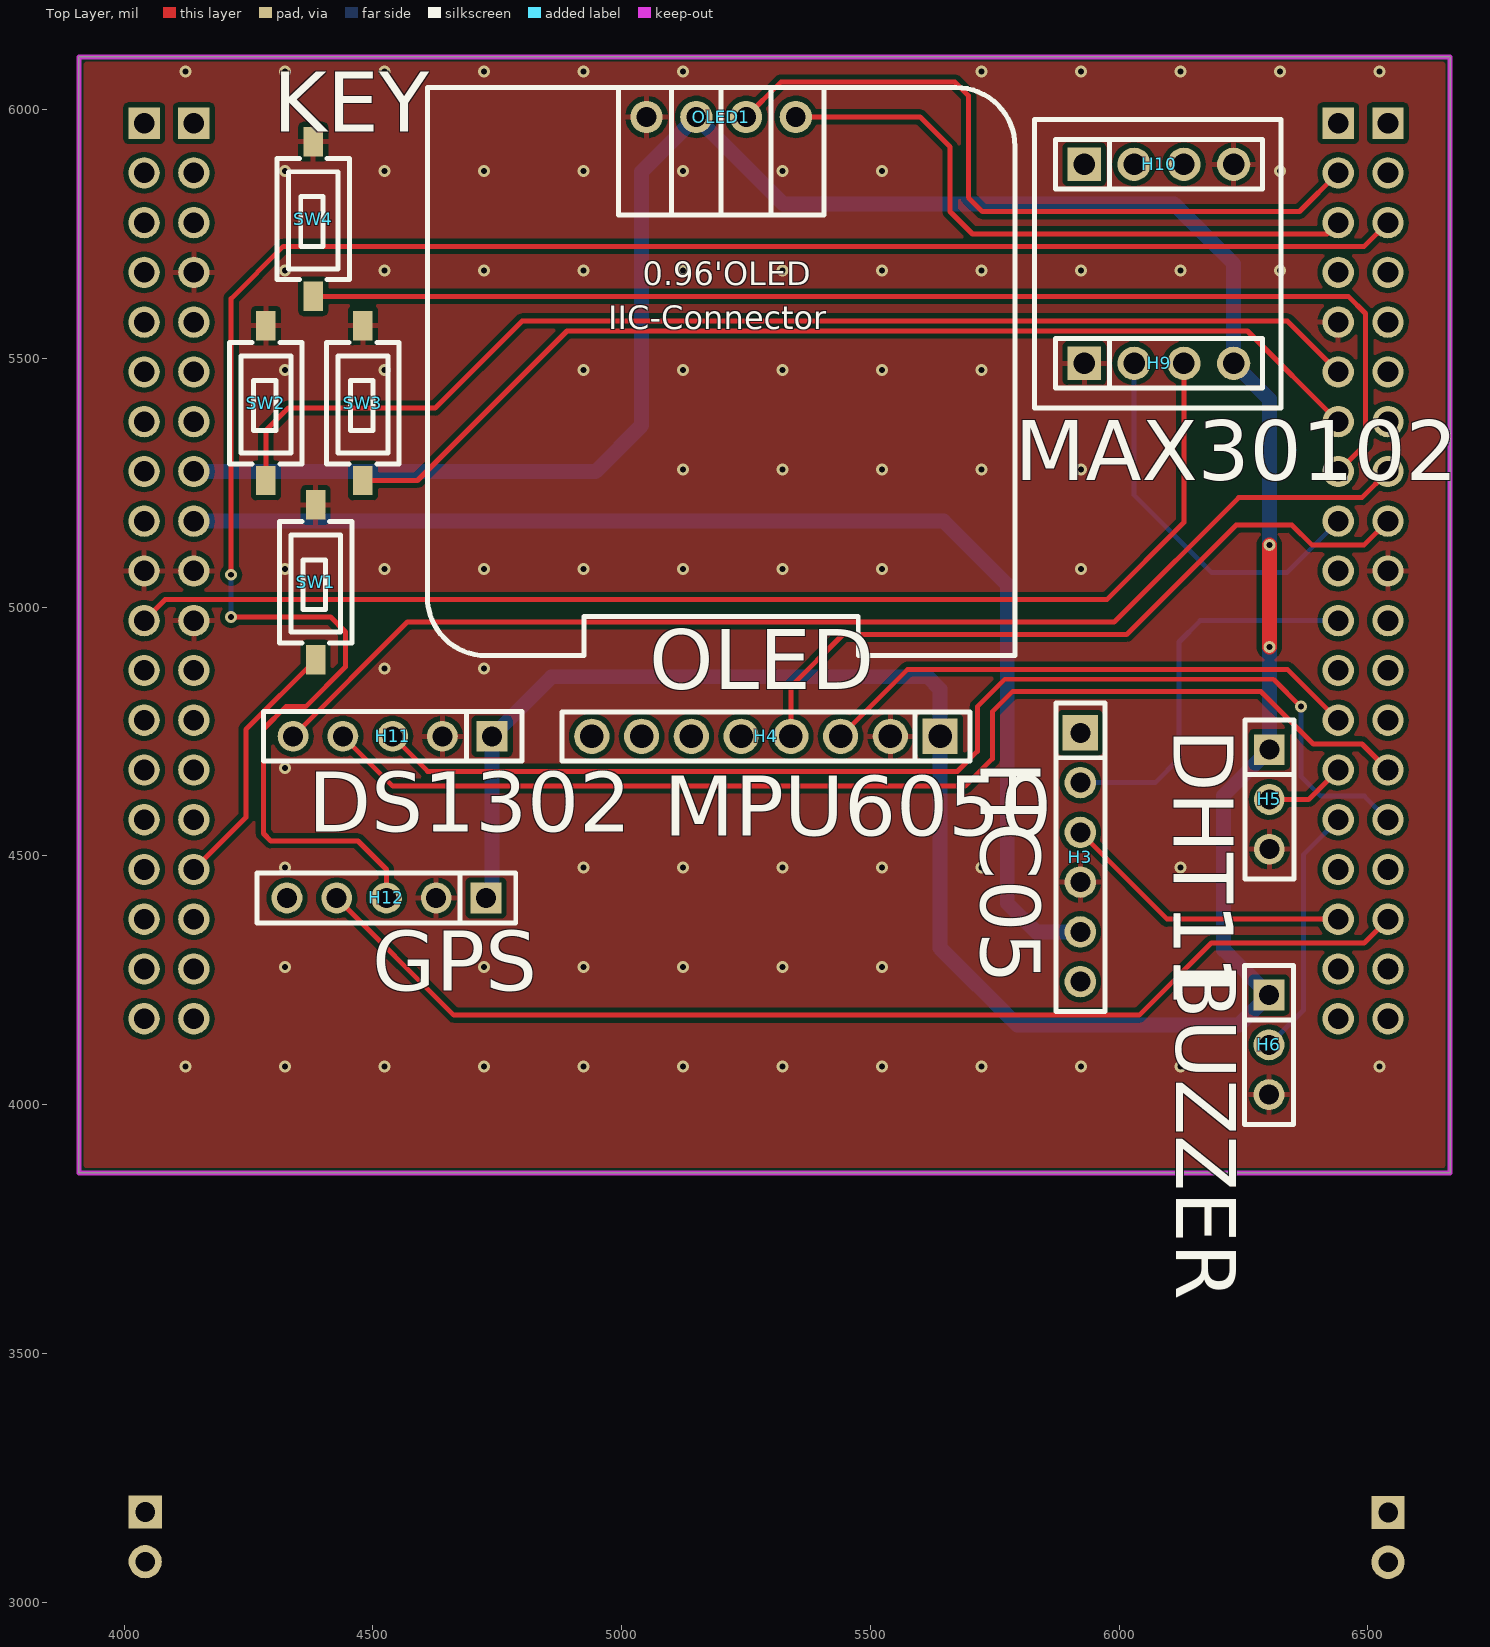
[diagram p0: Top Layer view]
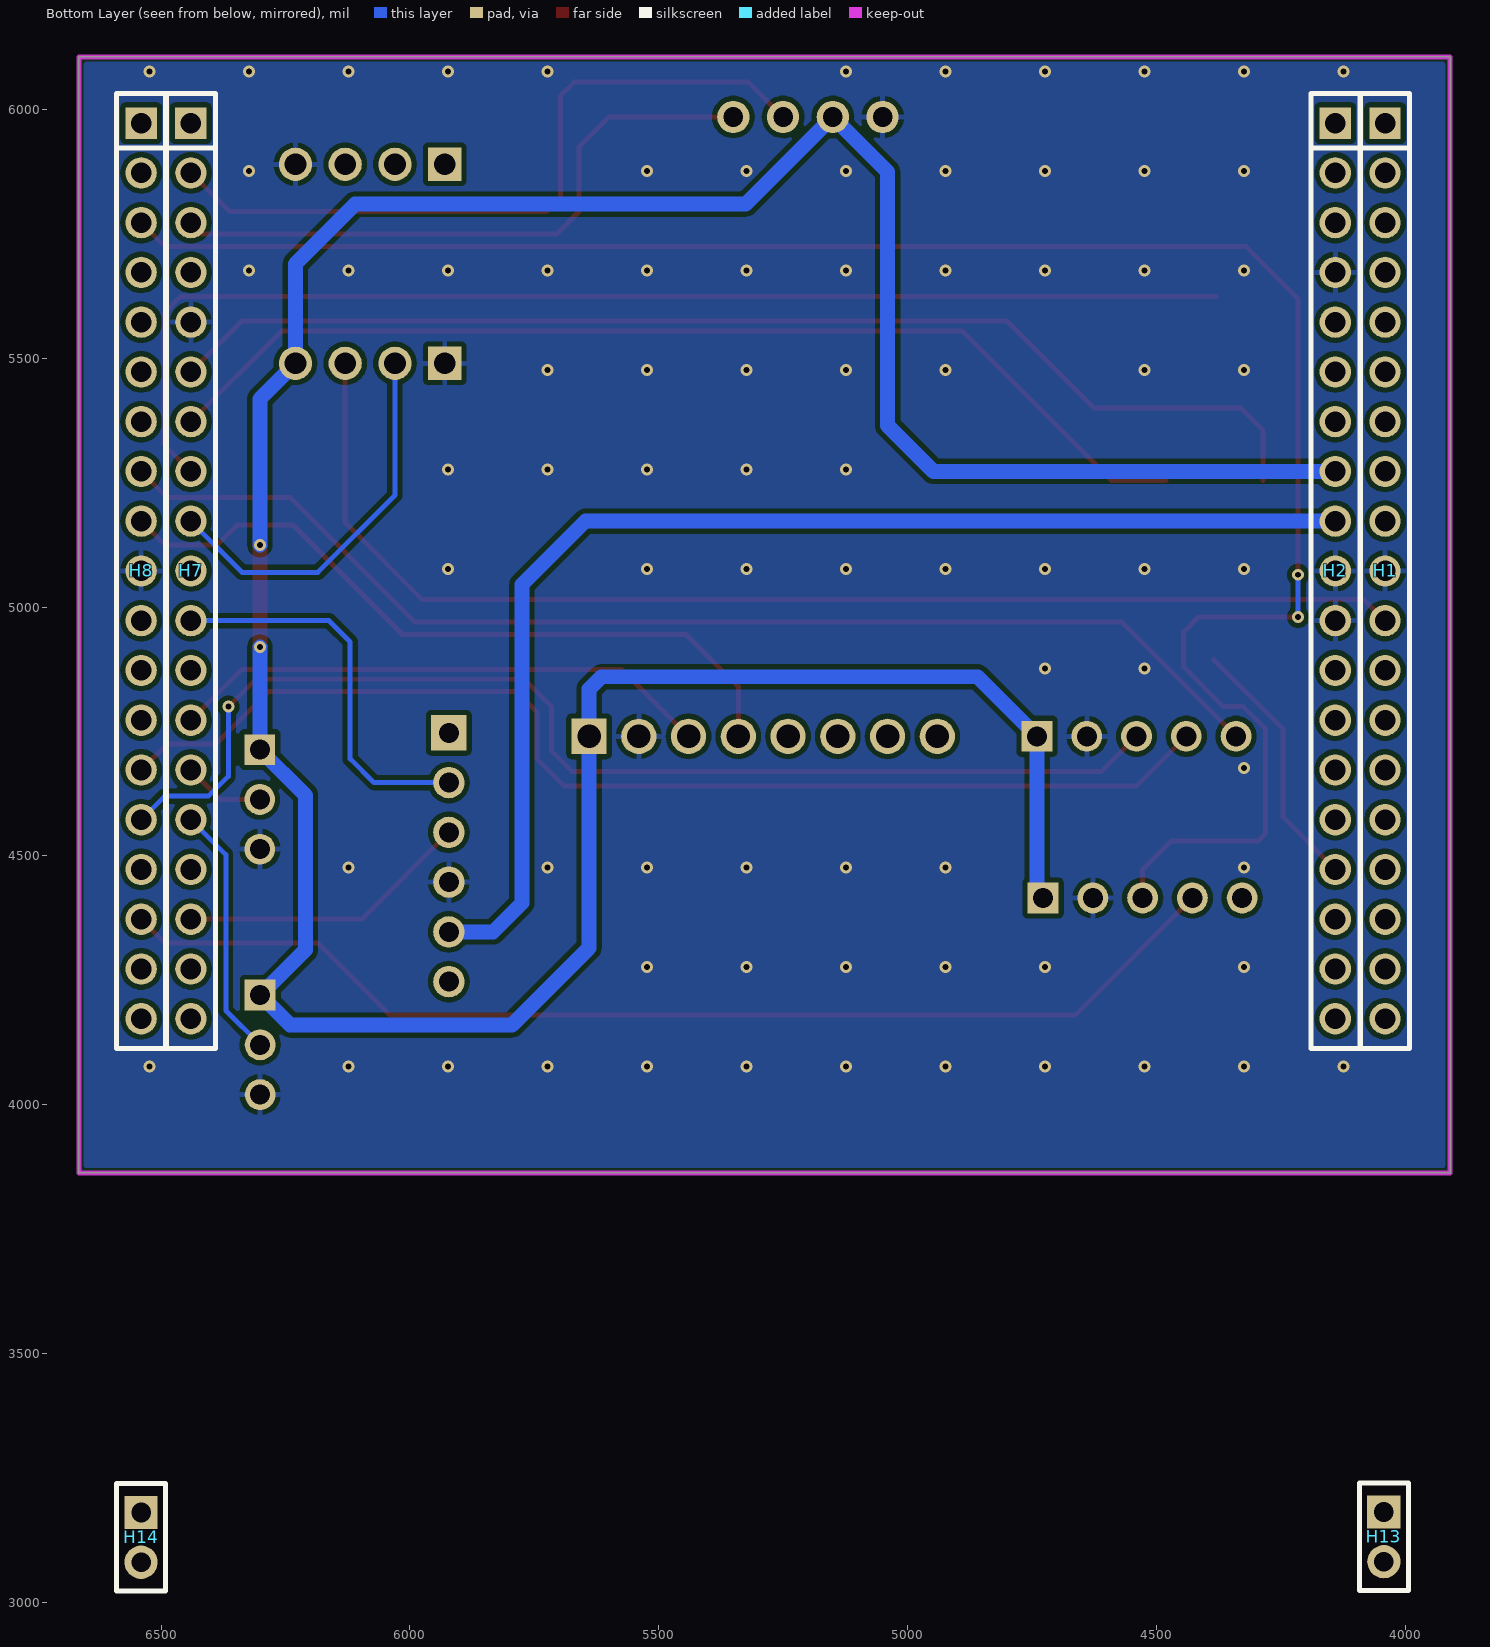
[diagram p1: Bottom Layer view, seen from below]
# Altium PCB MISC82907.pcbdoc
Units mil, origin at the board's own origin, x right, y up, seen from the top; angles counter-clockwise.
Board outline 2755.91 x 2243.03 mil, 2 copper layers (Top Layer, Bottom Layer), stack 62.206 mil thick; 19 components, 75 nets, 130 pads, 83 vias.

## Layer stack, top to bottom
Top Solder Mask Layer: solder mask 0.394, Dk 3.3
Top Layer: signal copper 1.379
Dielectric1: surface 59.449, FR4, Dk 4.5
Bottom Layer: signal copper 1.378
Bottom Solder Mask Layer: solder mask 0.394, Dk 3.3

## Board outline
6665.16,3862.65 6665.16,6105.69 3909.25,6105.69 3909.25,3862.65

## Design rules (kind name [scope] priority, off if disabled: settings)
BoardOutlineClearance copperThickness2oz_1 [All] p2 off: genericclearance=7.99 ignorepadtopadclearanceinfootprint=FALSE except(0: Arc-SplitContinuation Track-SplitContinuation SMDPad-SplitContinuation THPad-SplitContinuation Via-SplitContinuation Fill-SplitContinuation Region-SplitContinuation Poly-SplitContinuation Text-SplitContinuation Hole-SplitContinuation; 5.98: Arc-CutoutEdge SMDPad-CutoutEdge THPad-CutoutEdge Via-CutoutEdge Fill-CutoutEdge Region-CutoutEdge Text-CutoutEdge; 6.93: Hole-OutlineEdge Hole-CutoutEdge; 10: Poly-OutlineEdge Poly-CutoutEdge; 11.81: Arc-OutlineEdge Track-OutlineEdge SMDPad-OutlineEdge THPad-OutlineEdge Via-OutlineEdge Fill-OutlineEdge Region-OutlineEdge Text-OutlineEdge Track-CutoutEdge)
BoardOutlineClearance copperThickness1oz_1 [All] p4: genericclearance=4.02 ignorepadtopadclearanceinfootprint=FALSE except(0: Arc-SplitContinuation Track-SplitContinuation SMDPad-SplitContinuation THPad-SplitContinuation Via-SplitContinuation Fill-SplitContinuation Region-SplitContinuation Poly-SplitContinuation Text-SplitContinuation Hole-SplitContinuation; 6: SMDPad-CutoutEdge THPad-CutoutEdge Via-CutoutEdge Fill-CutoutEdge Region-CutoutEdge Text-CutoutEdge; 6.93: Hole-OutlineEdge Hole-CutoutEdge; 10: Poly-OutlineEdge Poly-CutoutEdge; 11.8: Arc-OutlineEdge Track-OutlineEdge SMDPad-OutlineEdge THPad-OutlineEdge Via-OutlineEdge Fill-OutlineEdge Region-OutlineEdge Text-OutlineEdge; 11.81: Arc-CutoutEdge Track-CutoutEdge)
Clearance copperThickness2oz [All] p1 off: gap=7.99 ignorepadtopadclearanceinfootprint=FALSE except(5.98: SMDPad-Track SMDPad-SMDPad THPad-Track SMDPad-THPad THPad-THPad Track-Via SMDPad-Via THPad-Via Via-Via Fill-Track Region-Track Fill-SMDPad Region-SMDPad Fill-THPad Region-THPad Fill-Via Region-Via Fill-Fill Fill-Region Region-Region Arc-Track Arc-SMDPad Arc-THPad Arc-Via Fill-Arc Region-Arc Arc-Arc Text-Track SMDPad-Text Text-THPad Text-Via Fill-Text Region-Text Arc-Text Text-Text; 6.93: Hole-Track Hole-SMDPad Hole-THPad Hole-Via Fill-Hole Region-Hole Hole-Arc Hole-Text; 10: Poly-Track Poly-SMDPad Poly-THPad Poly-Via Poly-Fill Poly-Region Poly-Poly Poly-Arc Poly-Text Poly-Hole)
Clearance copperThickness1oz [All] p3: gap=4.02 ignorepadtopadclearanceinfootprint=FALSE except(5.98: SMDPad-Track SMDPad-SMDPad THPad-Track SMDPad-THPad THPad-THPad Track-Via SMDPad-Via THPad-Via Via-Via Fill-Track Region-Track Fill-SMDPad Region-SMDPad Fill-THPad Region-THPad Fill-Via Region-Via Fill-Fill Fill-Region Region-Region; 6: Arc-Track Arc-SMDPad Arc-THPad Arc-Via Fill-Arc Region-Arc Arc-Arc Text-Track SMDPad-Text Text-THPad Text-Via Fill-Text Region-Text Arc-Text Text-Text; 6.93: Hole-Track Hole-SMDPad Hole-THPad Hole-Via Fill-Hole Region-Hole Hole-Arc Hole-Text; 10: Poly-Track Poly-SMDPad Poly-THPad Poly-Via Poly-Fill Poly-Region Poly-Poly Poly-Arc Poly-Text Poly-Hole)
DiffPairsRouting differentialPair [All] p1: maxlimit=6 minlimit=6 mostfreqgap=6 toplayer_minwidth=5 toplayer_prefwidth=10 toplayer_maxwidth=100 toplayer_mingap=6 toplayer_prefgap=6 toplayer_maxgap=6 bottomlayer_minwidth=5 bottomlayer_prefwidth=10 bottomlayer_maxwidth=100 bottomlayer_mingap=6 bottomlayer_prefgap=6 bottomlayer_maxgap=6 maxuncoupledlength=10
HoleToHoleClearance otherClearance [All] p1: gap=11.81 allowstackedmicrovias=TRUE
Length netLength [All] p1: minlimit=0 maxlimit=0
MatchedLengths netLengthTolerance [All] p1: tolerance=1000
PasteMaskExpansion pasteMaskExpansion [All] p1: expansion=0
PlaneConnect innerPlane [All] p1: planeconnectstyle=Relief reliefexpansion=20 reliefentries=4 reliefconductorwidth=10 reliefairgap=10
PolygonConnect copperRegion [(InNet('GND'))] p1: connectstyle=Relief reliefconductorwidth=10 reliefentries=4 polygonreliefangle="90 Angle" airgapwidth=10 via.connectstyle=Relief via.reliefconductorwidth=10 via.reliefentries=4 via.polygonreliefangle="90 Angle" via.airgapwidth=10
RoutingVias viaSize [All] p1: holewidth=12.01 width=24.02 viastyle="Through Hole" minholewidth=11.81 minwidth=19.68 maxholewidth=248.03 maxwidth=393.7
SolderMaskExpansion solderMaskExpansion [IsVia] p1: expansion=-1000 istentingtop=TRUE
SolderMaskExpansion solderMaskExpansion [All] p2: expansion=2 istentingtop=FALSE
Width copperThickness2oz_2 [All] p1 off: maxlimit=100 minlimit=8 preferedwidth=10
Width copperThickness1oz_2 [All] p2: maxlimit=100 minlimit=5 preferedwidth=10

## Components (designator, comment, footprint, x,y, rotation, side; value= is the part's Value field where it differs from the comment)
H1 "C2897382" HDR-TH_19P-P2.54-V-F 4040.16,5072.65 r270 bottom locked
H2 "C2897382" HDR-TH_19P-P2.54-V-F 4140.16,5072.65 r270 bottom locked
H3 "" HDR-TH_6P-P2.54-V-F 5921.75,4497.21 r270 top
H4 "" HDR-TH_8P-P2.54-V-F-1 5290,4740.21 r180 top
H5 "" HDR-TH_3P-P2.54-V-F 6301.67,4613.38 r270 top
H6 "" HDR-TH_3P-P2.54-V-F 6300.99,4120.2 r270 top
H7 "C2897382" HDR-TH_19P-P2.54-V-F 6440.16,5072.65 r270 bottom locked
H8 "C2897382" HDR-TH_19P-P2.54-V-F 6540.16,5072.65 r270 bottom locked
H9 "" HDR-TH_4P-P2.54-V-F 6080,5490 r0 top
H10 "" HDR-TH_4P-P2.54-V-F 6080,5890 r0 top
H11 "" HDR-TH_5P-P2.54-V-F 4539.61,4740.39 r180 top
H12 "" HDR-TH_5P-P2.54-V-F 4527.3,4415.39 r180 top
H13 "" HDR-TH_2P-P2.54-V-F 4042.44,3131.37 r270 bottom locked
H14 "" HDR-TH_2P-P2.54-V-F 6540.32,3130.31 r270 bottom locked
OLED1 "" 0.96OLED_4P 5200,5985 r0 top
SW1 "" Key_SMD_3.6x6.1x2.5 4385,5050 r90 top
SW2 "" Key_SMD_3.6x6.1x2.5 4285,5410 r90 top
SW3 "" Key_SMD_3.6x6.1x2.5 4480,5410 r90 top
SW4 "" Key_SMD_3.6x6.1x2.5 4380,5780 r90 top

## Footprints (in the part's own frame and the unit in brackets; to place one, negate y for a bottom-side part, rotate by r counter-clockwise, add the part's x,y. Pads: shape width x height; smd on the part's side, far side on the other; paste and mask are expansions set on the pad)
0.96OLED_4P [mm]
  round 1.65 hole 1 copper offset 0,0: 1(-3.81,-0.001) 2(-1.27,0.002) 3(1.27,0.002) 4(3.81,0.002)
  silkscreen extent -15,-27.5 15,1.5
HDR-TH_2P-P2.54-V-F [mm]
  rect 1.7x1.7 hole 1: 1(-1.27,0)
  round 1.7 hole 1: 2(1.27,0)
  silkscreen extent -2.74,-1.25 2.74,1.25
HDR-TH_3P-P2.54-V-F [mil]
  rect 62x62 hole 40.16: 1(-100,0)
  round 62 hole 40.16: 2(0,0) 3(100,0)
  silkscreen extent -160,-49 160,49
HDR-TH_4P-P2.54-V-F [mm]
  rect 1.7x1.7 hole 1.1: 1(-3.81,0)
  round 1.7 hole 1.1: 2(-1.27,0) 3(1.27,0) 4(3.81,0)
  silkscreen extent -5.29,-1.27 5.29,1.27
HDR-TH_5P-P2.54-V-F [mil]
  rect 62x62 hole 40.16: 1(-200,0)
  round 62 hole 40.16: 2(-100,0) 3(0,0) 4(100,0) 5(200,0)
  silkscreen extent -260,-50 260,50
HDR-TH_6P-P2.54-V-F [mm]
  rect 1.8x1.8 hole 1.02: 1(-6.35,0)
  round 1.6 hole 1.02: 2(-3.81,0) 3(-1.27,0) 4(1.27,0) 5(3.81,0) 6(6.35,0)
  silkscreen extent -7.87,-1.25 7.87,1.25
HDR-TH_8P-P2.54-V-F-1 [mm]
  rect 1.8x1.8 hole 1.2: 1(-8.89,0)
  round 1.8 hole 1.2: 2(-6.35,0) 3(-3.81,0) 4(-1.27,0) 5(1.27,0) 6(3.81,0) 7(6.35,0) 8(8.89,0)
  silkscreen extent -10.41,-1.25 10.41,1.25
HDR-TH_19P-P2.54-V-F [mm]
  rect 1.6x1.6 hole 1.05: 1(-22.86,0)
  round 1.6 hole 1.05: 2(-20.32,0) 3(-17.78,0) 4(-15.24,0) 5(-12.7,0) 6(-10.16,0) 7(-7.62,0) 8(-5.08,0) 9(-2.54,0) 10(0,0) 11(2.54,0) 12(5.08,0) 13(7.62,0) 14(10.16,0) 15(12.7,0) 16(15.24,0) 17(17.78,0) 18(20.32,0) 19(22.86,0)
  silkscreen extent -24.38,-1.25 24.38,1.25
Key_SMD_3.6x6.1x2.5 [mil]
  rect 59.1x39.4 smd paste+0 mask+2: 1(-155.5,0) 2(155.5,0)
  silkscreen extent -122,-73 122,73

## Via types
v1: diameter 24.02, hole 12, Top Layer to Bottom Layer, 83 vias

## Nets (pads, with @x,y where several pads share a name; then routed paths per layer and width w, separated by ;. In a path a pad name is that pad's centre, name@x,y a point inside that pad or via, vN(x,y) a via of type N, cw(c..) or ccw(c..) an arc to the next point about the centre after c; other vN are vias at no path point)
+3V3: H2.8 H4.1 H5.1 H6.1 H9.4 H11.1 H12.1 OLED1.2 | length 6941.6
  Top Layer w30: v1(6301.67,4920) v1(6301.67,5125)
  Bottom Layer w30: H2.8 4947.65,5272.65 5040,5365 5040,5875.05 5150,5985.05 5325.05,5810 6110,5810 6230,5690 H9.4 6301.67,5418.33 v1(6301.67,5125) ; H12.1 4739.61,4427.7 H11.1 4859.21,4860 5615,4860 5640,4835 H4.1 5640,4315 5795,4160 6240.79,4160 H6.1 6210,4311.18 6210,4621.71 H5.1 v1(6301.67,4920)
+5V: H2.9 H3.5 | length 2498.4
  Bottom Layer w30: H2.9 5647.35,5172.65 5775,5045 5775,4405 5832.79,4347.21 H3.5
ADO: H4.7
AGND: H8.16
AVDD: H7.4
BOOT0: H1.4
CLK: H8.15 H11.3 | length 2358
  Top Layer w10: H11.3 4610,4670 5675,4670 5715,4710 5715,4800 5770,4855 6310,4855 v1(6365,4800)
  Bottom Layer w10: v1(6365,4800) 6365,4660 6405,4620 6492.81,4620 H8.15
DAT: H8.14 H11.4 | length 2341.7
  Top Layer w10: H11.4 4540,4640 5690,4640 5745,4695 5745,4790 5785,4830 6285,4830 6390,4725 6487.81,4725 H8.14
E5V: H2.3
EN: H3.6
GND: H1.10 H2.4 H2.10 H2.11 H3.4 H4.2 H5.3 H6.3 H7.5 H8.10 H9.1 H10.4 H11.2 H12.2 OLED1.1 SW1.2 SW2.2 SW3.2 SW4.2
  other v1: 4123.35,4076.75 4323.35,4076.75 4523.35,4076.75 4723.35,4076.75 4923.35,4076.75 5123.35,4076.75 5323.35,4076.75 5523.35,4076.75 5723.35,4076.75 5923.35,4076.75 6123.35,4076.75 6523.35,4076.75 4323.35,4276.75 4723.35,4276.75 4923.35,4276.75 5123.35,4276.75 5323.35,4276.75 5523.35,4276.75 4323.35,4476.75 4923.35,4476.75 5123.35,4476.75 5323.35,4476.75 5523.35,4476.75 5723.35,4476.75 6123.35,4476.75 4323.35,4676.75 4523.35,4876.75 4723.35,4876.75 4323.35,5076.75 4523.35,5076.75 4723.35,5076.75 4923.35,5076.75 5123.35,5076.75 5323.35,5076.75 5523.35,5076.75 5923.35,5076.75 5123.35,5276.75 5323.35,5276.75 5523.35,5276.75 5723.35,5276.75 5923.35,5276.75 4323.35,5476.75 4523.35,5476.75 4923.35,5476.75 5123.35,5476.75 5323.35,5476.75 5523.35,5476.75 5723.35,5476.75 4323.35,5676.75 4523.35,5676.75 4723.35,5676.75 4923.35,5676.75 5123.35,5676.75 5323.35,5676.75 5523.35,5676.75 5723.35,5676.75 5923.35,5676.75 6123.35,5676.75 6323.35,5676.75 4323.35,5876.75 4523.35,5876.75 4723.35,5876.75 4923.35,5876.75 5123.35,5876.75 5323.35,5876.75 5523.35,5876.75 6323.35,5876.75 4123.35,6076.75 4323.35,6076.75 4523.35,6076.75 4723.35,6076.75 4923.35,6076.75 5123.35,6076.75 5723.35,6076.75 5923.35,6076.75 6123.35,6076.75 6323.35,6076.75 6523.35,6076.75
INT: H4.8
IOREF: H2.6
NC: H8.5
PA0: H2.14
PA1: H2.15
PA2: H7.18
PA3: H7.19
PA4: H2.16 SW1.1 | length 523.3
  Top Layer w10: H2.16 4245,4577.5 4245,4754.5 SW1.1
PA5: H7.6 SW2.1 | length 2389.2
  Top Layer w10: SW2.1 4285,5355 4330,5400 4625,5400 4800,5575 6337.81,5575 H7.6
PA6: H7.7 SW3.1 | length 2160.2
  Top Layer w10: SW3.1 4589.5,5254.5 4890,5555 6257.81,5555 H7.7
PA7: H7.8 SW4.1 | length 2469.4
  Top Layer w10: SW4.1 6460.5,5624.5 6495,5590 6495,5327.5 H7.8
PA8: H7.12
PA9: H3.2 H7.11 | length 790.9
  Bottom Layer w10: H3.2 6072.21,4647.21 6120,4695 6120,4930 6162.65,4972.65 H7.11
PA10: H3.3 H7.17 | length 590.7
  Top Layer w10: H3.3 6096.31,4372.65 H7.17
PA11: H8.7
PA12: H8.6
PA13: H1.7
PA14: H1.8
PA15: H1.9
PB0: H2.17
PB1: H8.12
PB2: H8.11
PB3: H7.16
PB4: H5.2 H7.14 | length 163
  Top Layer w10: H5.2 6380.89,4613.38 H7.14
PB5: H6.2 H7.15 | length 510.1
  Bottom Layer w10: H6.2 6370,4189.21 6370,4502.5 H7.15
PB6: H7.9 H9.2 | length 781.9
  Bottom Layer w10: H9.2 6030,5225 6185,5070 6337.5,5070 H7.9
PB7: H1.11 H9.3 | length 2491.7
  Top Layer w10: H1.11 4082.64,5015.14 4157.75,5015.14 4157.89,5015 5975,5015 6130,5170 H9.3
PB8: H7.2 OLED1.3 | length 1479.1
  Top Layer w10: OLED1.3@5250,5985.05 5319.95,6055 5670,6055 5697.18,6027.82 5697.18,5822.82 5725,5795 6362.5,5795 H7.2
PB9: H7.3 OLED1.4 | length 1273.1
  Top Layer w10: OLED1.4@5350,5985.05 5599.95,5985.05 5660,5925 5660,5795 5705,5750 6417.5,5750 H7.3
PB10: H4.3 H7.13 | length 1098.4
  Top Layer w10: H4.3 5574.79,4875 6337.81,4875 H7.13
PB11: H4.4 H8.9 | length 1470.9
  Top Layer w10: H4.4 5340,4840 5445,4945 6015,4945 6235,5165 6347.09,5165 6387.09,5125 6492.5,5125 H8.9
PB12: H8.8 H11.5 | length 2421
  Top Layer w10: H11.5 4569.21,4970 5990,4970 6240,5220 6487.5,5220 H8.8
PB15: H8.13
PC0: H2.19
PC1: H2.18
PC2: H1.18
PC3: H1.19
PC4: H8.17 H12.4 | length 2290.2
  Top Layer w10: H12.4 4662.7,4180 6040,4180 6185,4325 6492.5,4325 H8.17
PC5: H8.3 H12.3 | length 4102.1
  Top Layer w10: v1(4215,4980) 4415,4980 4445,4950 4445,4880 4365,4800 4325,4800 4280,4755 4280,4545 4295,4530 4470,4530 4527.3,4472.7 H12.3 ; v1(4215,5065) 4215,5620 4320,5725 6492.5,5725 H8.3
  Bottom Layer w10: v1(4215,4980) v1(4215,5065)
PC6: H8.2
PC7: H7.10
PC8: H8.1
PC9: H7.1
PC10: H1.1
PC11: H2.1
PC12: H1.2
PC13: H1.12
PC14: H1.13
PC15: H1.14
PD2: H2.2
PF0: H1.15
PF1: H1.16
PF4: H8.19
PF5: H8.18
PF6: H1.5
PF7: H1.6
RESET: H2.7
STATE: H3.1
U5V: H8.4
VBAT: H1.17
VDD: H1.3
VIN: H2.12
XCL: H4.6
XDA: H4.5
pads on no net: H2.5 H2.13 H10.1 H10.2 H10.3 H12.5 H13.1 H13.2 H14.1 H14.2

## Polygon pours and split planes (outlines as drawn)
GND on Bottom Layer (solid, remove dead copper, pour order 2): 3750,6335 3750,3735 6825,3735 6825,6335
GND on Top Layer (solid, remove dead copper, pour order 0): 3715,6305 3715,3750 6870,3750 6870,6305

## Keep-outs
Board Outline Layer:
  the board outline again, w10

## Silkscreen, mask and mechanical layers (free items; w line width, h text height)
Top Silkscreen Layer:
  lines w10: 5830,5400 5830,5980 6325,5980 6325,5400 5830,5400
  text "KEY" at 4300,5955 h120
  text "MAX30102" at 5790,5255 h120
  text "OLED" at 5055,4835 h120
  text "DHT11" at 6110,4755 h120 r270
  text "HC05" at 5721.54,4691.51 h120 r270
  text "DS1302" at 4370,4548.28 h120
  text "MPU6050" at 5085,4540 h120
  text "BUZZER" at 6114.8,4285.2 h120 r270
  text "GPS" at 4498.91,4228.91 h120